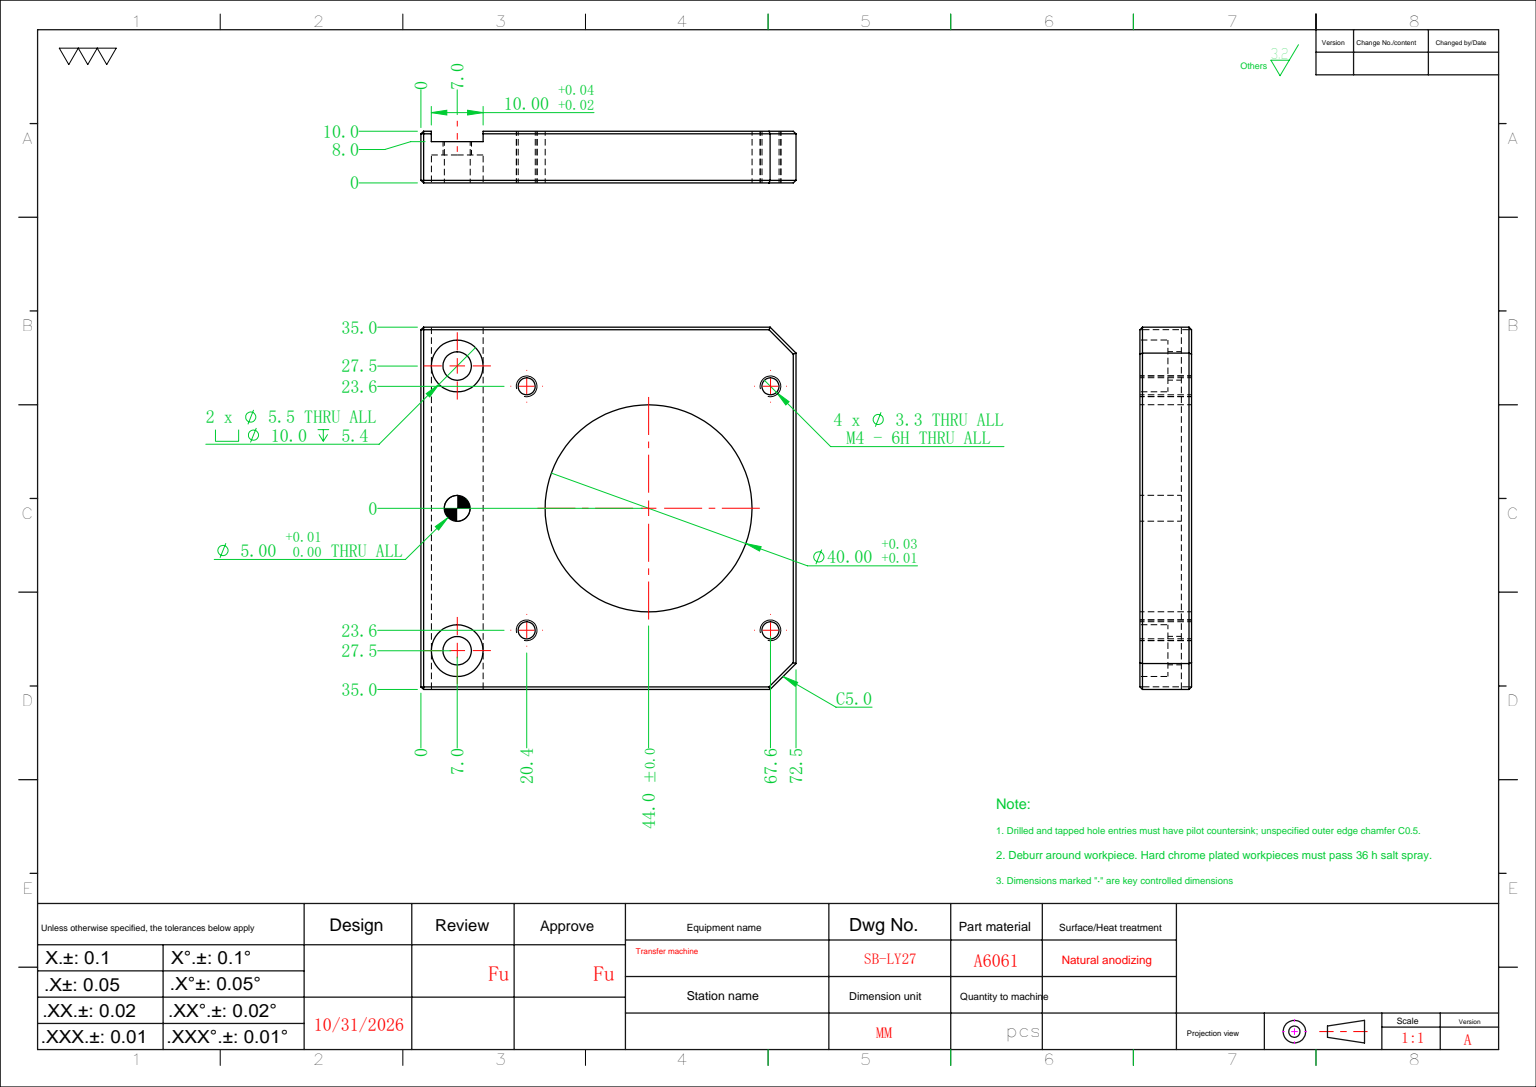
SolidWorks part; units mm, degrees
ref_plane "前视基准面" through (0, 0, 0) normal (0, 0, 1) x (1, 0, 0)
ref_plane "上视基准面" through (0, 0, 0) normal (0, 1, 0) x (1, 0, 0)
ref_plane "右视基准面" through (0, 0, 0) normal (1, 0, 0) x (0, 0, -1)
sketch "草图1" plane through (0, 0, 0) normal (0, 0, 1) x (1, 0, 0)
  line L1 (-35, -36.25) -> (35, -36.25)
  line L2 (-35, -36.25) -> (-35, 36.25)
  line L3 (-35, 36.25) -> (35, 36.25)
  line L4 (35, -36.25) -> (35, 36.25)
  line L5 (-35, -36.25) -> (35, 36.25) construction
  line L6 (-35, 36.25) -> (35, -36.25) construction
  point P0 (0, 0)
  dimension "D1" = 70
  dimension "D2" = 72.5
extrude "凸台-拉伸1" add sketch "草图1" along normal blind 10
sketch "草图2" plane through (-35, 0, 0) normal (-1, 0, 0) x (0, 0, 1)
  line L0 (0, 36.25) -> (0, -36.25) construction
  line L1 (0, 34.25) -> (2, 34.25)
  line L2 (0, 34.25) -> (0, 24.25)
  line L3 (0, 24.25) -> (2, 24.25)
  line L4 (2, 34.25) -> (2, 24.25)
  line L5 (10, 36.25) -> (0, 36.25) construction
  dimension "D1" = 10
  dimension "D2" = 2
  dimension "D3" = 2
extrude "切除-拉伸1" cut sketch "草图2" against normal through all
hole_wizard "M5 六角凹头螺钉的柱形沉头孔1" positions "草图3" profile "草图4" counterbore size "M5" standard "ISO" end condition through all
sketch "草图3" plane through (0, 0, 10) normal (0, 0, 1) x (1, 0, 0)
  line L0 (-35, 29.25) -> (35, 29.25) construction
  line L1 (-35, 24.25) -> (-35, 34.25) construction
  line L2 (35, 24.25) -> (35, 34.25) construction
  line L4 (0, 0) -> (0, 44.0272) construction
  point P0 (27.5, 29.25)
  point P2 (-27.5, 29.25)
  dimension "D1" = 55
sketch "草图4" plane through (27.5, 29.25, 10) normal (1, 0, 0) x (0, -1, 0)
  line L0 (0, 0) -> (0, 10)
  line L1 (0, 10) -> (2.75, 10)
  line L3 (2.75, 10) -> (2.75, 5.4)
  line L4 (2.75, 5.4) -> (5, 5.4)
  line L5 (5, 5.4) -> (5, 0)
  line L7 (5, 0) -> (0, 0)
  line L11 (0, -6.35) -> (0, 107.95) construction
  dimension "通孔孔直径" = 5.5
  dimension "通孔孔深度" = 10
  dimension "柱形沉头孔直径" = 10
  dimension "柱形沉头孔深度" = 5.4
hole_wizard "大小mm 暗销孔1" positions "草图5" profile "草图6" hole size "Ø5.0" standard "ISO" end condition through all
sketch "草图5" plane through (0, 0, 10) normal (0, 0, 1) x (1, 0, 0)
  line L0 (27.5, 29.25) -> (-27.5, 29.25) construction
  point P0 (0, 29.25)
sketch "草图6" plane through (0, 29.25, 10) normal (1, 0, 0) x (0, -1, 0)
  line L0 (0, 0) -> (0, 10)
  line L1 (0, 10) -> (2.5, 10)
  line L2 (2.5, 10) -> (2.5, 0)
  line L5 (2.5, 0) -> (0, 0)
  line L11 (0, -6.35) -> (0, 107.95) construction
  dimension "通孔孔直径" = 5
  dimension "通孔孔深度" = 10
hole_wizard "M4 螺纹孔1" positions "草图7" profile "草图8" tap size "M4" standard "ISO" end condition through all
sketch "草图7" plane through (0, 0, 10) normal (0, 0, 1) x (1, 0, 0)
  line L1 (-23.57, 15.82) -> (23.57, 15.82) construction
  line L2 (-23.57, 15.82) -> (-23.57, -31.32) construction
  line L3 (-23.57, -31.32) -> (23.57, -31.32) construction
  line L4 (23.57, 15.82) -> (23.57, -31.32) construction
  line L5 (23.57, -7.75) -> (-23.57, -7.75) construction
  line L7 (0, -31.32) -> (0, 15.82) construction
  line L9 (35, 36.25) -> (-35, 36.25) construction
  point P0 (-23.57, 15.82)
  point P3 (-23.57, -31.32)
  point P6 (23.57, -31.32)
  point P9 (23.57, 15.82)
  dimension "D1" = 47.14
  dimension "D2" = 44
sketch "草图8" plane through (-23.57, 15.82, 10) normal (1, 0, 0) x (0, -1, 0)
  line L0 (0, 0) -> (0, 10)
  line L1 (0, 10) -> (1.65, 10)
  line L2 (1.65, 10) -> (1.65, 0)
  line L5 (1.65, 0) -> (0, 0)
  line L11 (0, -6.35) -> (0, 107.95) construction
  dimension "通孔螺纹孔钻头直径" = 3.3
  dimension "通孔螺纹孔钻头深度" = 10
cosmetic thread "孔螺蚊线1" parameters "D2"=4
cosmetic thread "孔螺蚊线2" parameters "D2"=4
cosmetic thread "孔螺蚊线3" parameters "D2"=4
cosmetic thread "孔螺蚊线4" parameters "D2"=4
sketch "草图9" plane through (0, 0, 0) normal (0, 0, -1) x (-1, 0, 0)
  line L0 (-23.57, 15.82) -> (23.57, 15.82) construction
  line L1 (23.57, -31.32) -> (-23.57, -31.32) construction
  line L2 (0, -31.32) -> (0, 15.82) construction
  circle A0 centre (0, -7.75) radius 20
  dimension "D1" = 40
extrude "切除-拉伸2" cut sketch "草图9" against normal through all
chamfer "倒角1" distance 5 angle 45 2 edges at (35, -36.25, 5) (-35, -36.25, 5)
chamfer "倒角2" distance 0.5 angle 45 16 edges at (-35, -3.5, 0) (-32.5, -33.75, 0) (0, -36.25, 0) (32.5, -33.75, 0) (35, -3.5, 0) (-32.5, -33.75, 10) (-35, 2.5, 10) (0, -36.25, 10) (32.5, -33.75, 10) (35, 2.5, 10) (35, 36.25, 5) (0, 36.25, 10) (-35, 36.25, 5) (-35, 35.25, 0) (0, 36.25, 0) (35, 35.25, 0)
